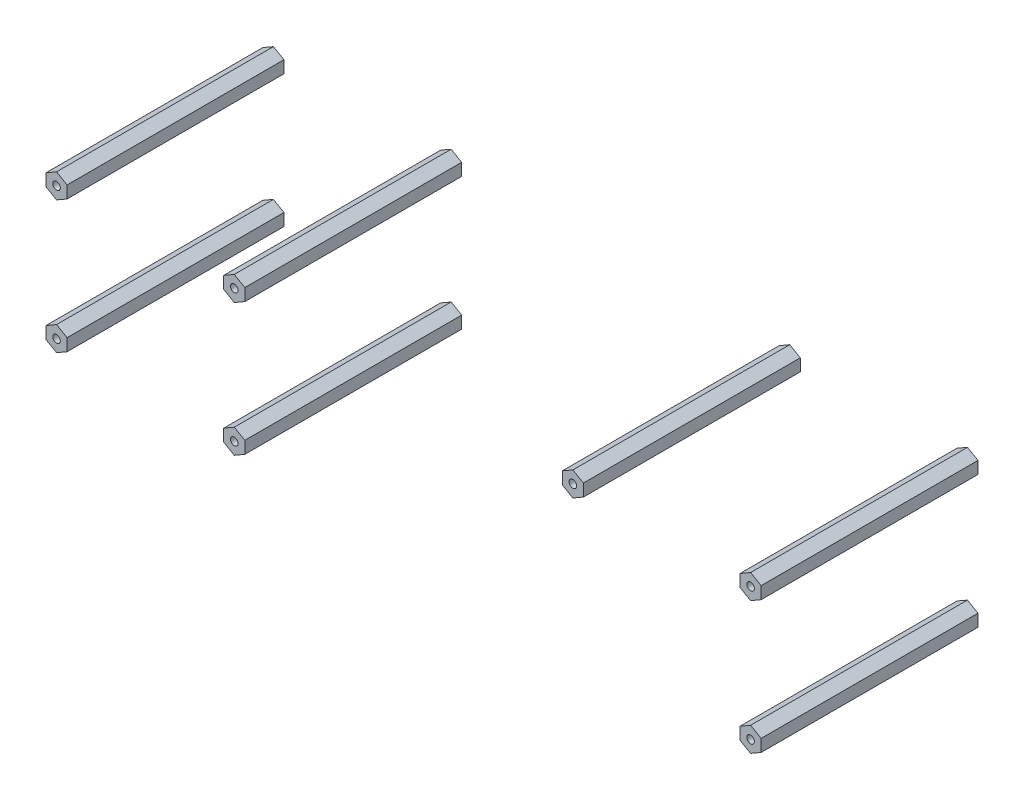
from build123d import *

# Parameters (mm, degrees)
BOSS_EXTRUDE1_DEPTH        = 70
BOSS_EXTRUDE1_DEPTH_BACK   = 2
BOSS_EXTRUDE1_2_DEPTH      = 70
BOSS_EXTRUDE1_2_DEPTH_BACK = 2
BOSS_EXTRUDE1_3_DEPTH      = 70
BOSS_EXTRUDE1_3_DEPTH_BACK = 2
BOSS_EXTRUDE1_4_DEPTH      = 70
BOSS_EXTRUDE1_4_DEPTH_BACK = 2
BOSS_EXTRUDE1_5_DEPTH      = 70
BOSS_EXTRUDE1_5_DEPTH_BACK = 2
BOSS_EXTRUDE1_6_DEPTH      = 70
BOSS_EXTRUDE1_6_DEPTH_BACK = 2
BOSS_EXTRUDE1_7_DEPTH      = 70
BOSS_EXTRUDE1_7_DEPTH_BACK = 2
M3_TAPPED_HOLE1_AT_2_COUNT = 2
M3_TAPPED_HOLE1_AT_2_PITCH = 44
M3_TAPPED_HOLE1_AT_3_COUNT = 2
M3_TAPPED_HOLE1_AT_3_PITCH = 73.600271739
M3_TAPPED_HOLE1_AT_4_COUNT = 2
M3_TAPPED_HOLE1_AT_4_PITCH = 59
M3_TAPPED_HOLE1_AT_5_COUNT = 2
M3_TAPPED_HOLE1_AT_5_PITCH = 176.957509024
M3_TAPPED_HOLE1_AT_6_COUNT = 2
M3_TAPPED_HOLE1_AT_6_PITCH = 234.563765318
M3_TAPPED_HOLE1_AT_7_COUNT = 2
M3_TAPPED_HOLE1_AT_7_PITCH = 230.4


with BuildPart() as part:
    # Sketch1 → Boss-Extrude1 (new, two sides: drawn at the far end of the back side and taken through both)
    with BuildSketch(Plane.XY.offset(-BOSS_EXTRUDE1_DEPTH_BACK)):
        Polygon((118.7, -6.020725942), (115.2, -4), (111.7, -6.020725942), (111.7, -10.062177826), (115.2, -12.082903769), (118.7, -10.062177826), align=None)
    extrude(amount=BOSS_EXTRUDE1_DEPTH + BOSS_EXTRUDE1_DEPTH_BACK)


with BuildPart() as body_2:
    # Sketch1 → Boss-Extrude1 2 (new, two sides: drawn at the far end of the back side and taken through both)
    with BuildSketch(Plane.XY.offset(-BOSS_EXTRUDE1_2_DEPTH_BACK)):
        Polygon((59.7, -6.020725942), (56.2, -4), (52.7, -6.020725942), (52.7, -10.062177826), (56.2, -12.082903769), (59.7, -10.062177826), align=None)
    extrude(amount=BOSS_EXTRUDE1_2_DEPTH + BOSS_EXTRUDE1_2_DEPTH_BACK)


with BuildPart() as body_3:
    # Sketch1 → Boss-Extrude1 3 (new, two sides: drawn at the far end of the back side and taken through both)
    with BuildSketch(Plane.XY.offset(-BOSS_EXTRUDE1_3_DEPTH_BACK)):
        Polygon((118.7, -49.937822174), (118.7, -53.979274058), (115.2, -56), (111.7, -53.979274058), (111.7, -49.937822174), (115.2, -47.917096231), align=None)
    extrude(amount=BOSS_EXTRUDE1_3_DEPTH + BOSS_EXTRUDE1_3_DEPTH_BACK)


with BuildPart() as body_4:
    # Sketch1 → Boss-Extrude1 4 (new, two sides: drawn at the far end of the back side and taken through both)
    with BuildSketch(Plane.XY.offset(-BOSS_EXTRUDE1_4_DEPTH_BACK)):
        Polygon((-118.7, -53.979274058), (-115.2, -56), (-111.7, -53.979274058), (-111.7, -49.937822174), (-115.2, -47.917096231), (-118.7, -49.937822174), align=None)
    extrude(amount=BOSS_EXTRUDE1_4_DEPTH + BOSS_EXTRUDE1_4_DEPTH_BACK)

    # Sketch3 → M3 Tapped Hole1 (revolve, cut)
    with BuildSketch(Plane(origin=(-115.2, -52, 70), x_dir=(0, -1, 0), z_dir=(1, 0, 0))):
        Polygon((0, 0), (0, 9.251075774), (1.25, 8.5), (1.25, 0), align=None)
    m3_tapped_hole1 = revolve(axis=Axis((-115.2, -52, 76.35), (0, 0, -1)), mode=Mode.SUBTRACT)


with BuildPart() as body_5:
    # Sketch1 → Boss-Extrude1 5 (new, two sides: drawn at the far end of the back side and taken through both)
    with BuildSketch(Plane.XY.offset(-BOSS_EXTRUDE1_5_DEPTH_BACK)):
        Polygon((-118.7, -10.062177826), (-118.7, -6.020725942), (-115.2, -4), (-111.7, -6.020725942), (-111.7, -10.062177826), (-115.2, -12.082903769), align=None)
    extrude(amount=BOSS_EXTRUDE1_5_DEPTH + BOSS_EXTRUDE1_5_DEPTH_BACK)

    # M3 Tapped Hole1 at 2: M3 Tapped Hole1 ×2
    with Locations(*[(0, i * M3_TAPPED_HOLE1_AT_2_PITCH, 0) for i in range(1, M3_TAPPED_HOLE1_AT_2_COUNT)]):
        add(m3_tapped_hole1, mode=Mode.SUBTRACT)


with BuildPart() as body_6:
    # Sketch1 → Boss-Extrude1 6 (new, two sides: drawn at the far end of the back side and taken through both)
    with BuildSketch(Plane.XY.offset(-BOSS_EXTRUDE1_6_DEPTH_BACK)):
        Polygon((-59.7, -10.062177826), (-59.7, -6.020725942), (-56.2, -4), (-52.7, -6.020725942), (-52.7, -10.062177826), (-56.2, -12.082903769), align=None)
    extrude(amount=BOSS_EXTRUDE1_6_DEPTH + BOSS_EXTRUDE1_6_DEPTH_BACK)

    # M3 Tapped Hole1 at 3: M3 Tapped Hole1 ×2
    with Locations(*[Vector(0.8016274750930587, 0.5978238797304166, 0) * (i * M3_TAPPED_HOLE1_AT_3_PITCH) for i in range(1, M3_TAPPED_HOLE1_AT_3_COUNT)]):
        add(m3_tapped_hole1, mode=Mode.SUBTRACT)


with BuildPart() as body_7:
    # Sketch1 → Boss-Extrude1 7 (new, two sides: drawn at the far end of the back side and taken through both)
    with BuildSketch(Plane.XY.offset(-BOSS_EXTRUDE1_7_DEPTH_BACK)):
        Polygon((-59.7, -53.979274058), (-56.2, -56), (-52.7, -53.979274058), (-52.7, -49.937822174), (-56.2, -47.917096231), (-59.7, -49.937822174), align=None)
    extrude(amount=BOSS_EXTRUDE1_7_DEPTH + BOSS_EXTRUDE1_7_DEPTH_BACK)

    # M3 Tapped Hole1 at 4: M3 Tapped Hole1 ×2
    with Locations(*[(i * M3_TAPPED_HOLE1_AT_4_PITCH, 0, 0) for i in range(1, M3_TAPPED_HOLE1_AT_4_COUNT)]):
        add(m3_tapped_hole1, mode=Mode.SUBTRACT)


with BuildPart() as body_2_1:
    add(body_2.part)

    # M3 Tapped Hole1 at 5: M3 Tapped Hole1 ×2
    with Locations(*[Vector(0.9685941045694556, 0.24864726138305773, 0) * (i * M3_TAPPED_HOLE1_AT_5_PITCH) for i in range(1, M3_TAPPED_HOLE1_AT_5_COUNT)]):
        add(m3_tapped_hole1, mode=Mode.SUBTRACT)


with BuildPart() as part_1:
    add(part.part)

    # M3 Tapped Hole1 at 6: M3 Tapped Hole1 ×2
    with Locations(*[Vector(0.9822488980255548, 0.1875822548312693, 0) * (i * M3_TAPPED_HOLE1_AT_6_PITCH) for i in range(1, M3_TAPPED_HOLE1_AT_6_COUNT)]):
        add(m3_tapped_hole1, mode=Mode.SUBTRACT)


with BuildPart() as body_3_1:
    add(body_3.part)

    # M3 Tapped Hole1 at 7: M3 Tapped Hole1 ×2
    with Locations(*[(i * M3_TAPPED_HOLE1_AT_7_PITCH, 0, 0) for i in range(1, M3_TAPPED_HOLE1_AT_7_COUNT)]):
        add(m3_tapped_hole1, mode=Mode.SUBTRACT)


solid = Compound([body_4.part, body_5.part, body_6.part, body_7.part, body_2_1.part, part_1.part, body_3_1.part])
